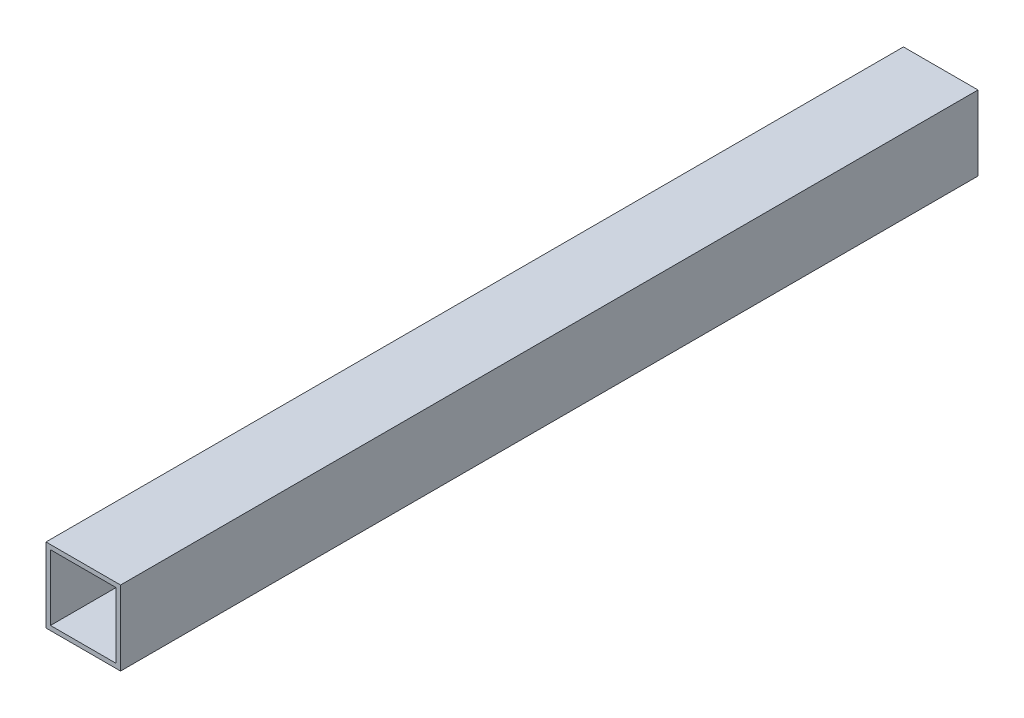
SolidWorks part; units mm, degrees
ref_plane "前视基准面" through (0, 0, 0) normal (0, 0, 1) x (1, 0, 0)
ref_plane "上视基准面" through (0, 0, 0) normal (0, 1, 0) x (1, 0, 0)
ref_plane "右视基准面" through (0, 0, 0) normal (1, 0, 0) x (0, 0, -1)
sketch "草图1" plane through (0, 0, 0) normal (0, 0, 1) x (1, 0, 0)
  line L0 (0, 0) -> (0, 50)
  line L1 (0, 50) -> (50, 50)
  line L2 (50, 50) -> (50, 0)
  line L3 (50, 0) -> (0, 0)
  line L4 (3, 3) -> (3, 47)
  line L5 (3, 47) -> (47, 47)
  line L6 (47, 47) -> (47, 3)
  line L7 (47, 3) -> (3, 3)
  dimension "D1" = 3
extrude "凸台-拉伸1" add sketch "草图1" along normal blind 600
sketch "草图2" plane through (0, 0, 600) normal (0, 0, 1) x (1, 0, 0)
  line L4 (3, 47) -> (3, 3)
  line L5 (3, 3) -> (47, 3)
  line L6 (47, 3) -> (47, 47)
  line L7 (47, 47) -> (3, 47)
  line L8 (0, 0) -> (50, 0)
  line L9 (50, 0) -> (50, 50)
  line L10 (50, 50) -> (0, 50)
  line L11 (0, 50) -> (0, 0)
  line L12 (0, 0) -> (50, 0)
  line L13 (50, 0) -> (50, 50)
  line L14 (50, 50) -> (0, 50)
  line L15 (0, 50) -> (0, 0)
  dimension "D1" = 0
extrude "切除-拉伸1" cut sketch "草图2" against normal blind 25
